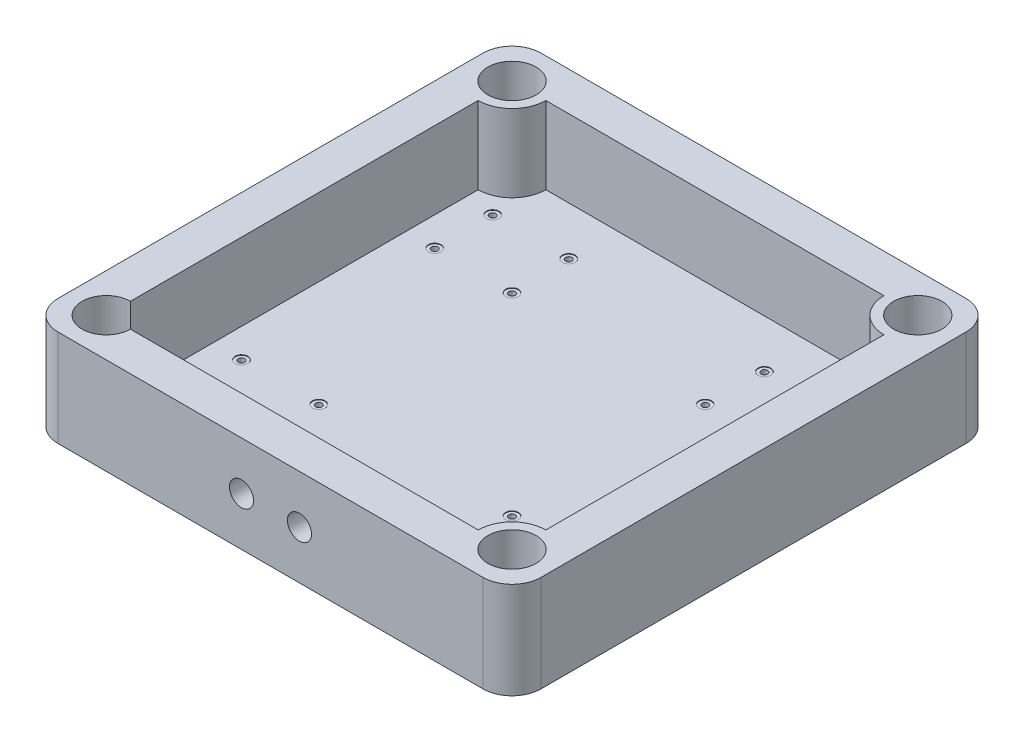
from build123d import *

# Parameters (mm, degrees)
BOSS_EXTRUDE1_DEPTH                          = 100
CUT_EXTRUDE1_DEPTH                           = 80
SKETCH3_R                                    = 25
CUT_EXTRUDE2_DEPTH                           = 80
SKETCH10_R                                   = 12.5
CUT_EXTRUDE4_DEPTH                           = 40
CBORE_FOR_M6_HEXAGON_HEAD_BOLTS_FULL_2_COUNT = 2
CBORE_FOR_M6_HEXAGON_HEAD_BOLTS_FULL_2_PITCH = 80
CBORE_FOR_M6_HEXAGON_HEAD_BOLTS_FULL_3_COUNT = 2
CBORE_FOR_M6_HEXAGON_HEAD_BOLTS_FULL_3_PITCH = 60
CBORE_FOR_M6_HEXAGON_HEAD_BOLTS_FULL_4_COUNT = 2
CBORE_FOR_M6_HEXAGON_HEAD_BOLTS_FULL_4_PITCH = 98.990867508
CUT_EXTRUDE5_DEPTH                           = 80


with BuildPart() as part:
    # Sketch1 → Boss-Extrude1 (new body)
    with BuildSketch(Plane(origin=(0, 0, 0), x_dir=(1, 0, 0), z_dir=(0, 1, 0))):
        with BuildLine():
            Line((-220, -250), (220, -250))
            ThreePointArc((220, -250), (241.213203436, -241.213203436), (250, -220))
            Line((250, -220), (250, 220))
            ThreePointArc((250, 220), (241.213203436, 241.213203436), (220, 250))
            Line((220, 250), (-220, 250))
            ThreePointArc((-220, 250), (-241.213203436, 241.213203436), (-250, 220))
            Line((-250, 220), (-250, -220))
            ThreePointArc((-250, -220), (-241.213203436, -241.213203436), (-220, -250))
        make_face()
    extrude(amount=BOSS_EXTRUDE1_DEPTH)

    # Sketch2 → Cut-Extrude1 (cut)
    with BuildSketch(Plane(origin=(0, 100, 0), x_dir=(1, 0, 0), z_dir=(0, 1, 0))):
        with BuildLine():
            Line((-175, -210), (175, -210))
            ThreePointArc((175, -210), (185.251262658, -185.251262658), (210, -175))
            Line((210, -175), (210, 175))
            ThreePointArc((210, 175), (185.251262658, 185.251262658), (175, 210))
            Line((175, 210), (-175, 210))
            ThreePointArc((-175, 210), (-185.251262658, 185.251262658), (-210, 175))
            Line((-210, 175), (-210, -175))
            ThreePointArc((-210, -175), (-185.251262658, -185.251262658), (-175, -210))
        make_face()
    extrude(amount=-CUT_EXTRUDE1_DEPTH, mode=Mode.SUBTRACT)

    # Sketch3 → Cut-Extrude2 (cut)
    with BuildSketch(Plane(origin=(0, 100, 0), x_dir=(1, 0, 0), z_dir=(0, 1, 0))):
        with Locations(Location((-210, 210, 0), (0, 0, 270))):
            Circle(SKETCH3_R)
        with Locations(Location((210, 210, 0), (0, 0, 90))):
            Circle(SKETCH3_R)
        with Locations(Location((210, -210, 0), (0, 0, 270))):
            Circle(SKETCH3_R)
        with Locations(Location((-210, -210, 0), (0, 0, 90))):
            Circle(SKETCH3_R)
    extrude(amount=-CUT_EXTRUDE2_DEPTH, mode=Mode.SUBTRACT)

    # Sketch10 → Cut-Extrude4 (cut)
    with BuildSketch(Plane.XY.offset(250)):
        with Locations((-30, 50)):
            Circle(SKETCH10_R)
        with Locations((30, 50)):
            Circle(SKETCH10_R)
    extrude(amount=-CUT_EXTRUDE4_DEPTH, mode=Mode.SUBTRACT)

    # Sketch12 → CBORE for M6 Hexagon head bolts-Full thread-grade C1 (revolve, cut)
    with BuildSketch(Plane(origin=(-180, 20, 100), x_dir=(0, 0, 1), z_dir=(1, 0, 0))):
        Polygon((0, 0), (0, 20), (3.3, 20), (3.3, 0.5), (6.5, 0.5), (6.5, 0.025), (6.525, 0), align=None)
    cbore_for_m6_hexagon_head_bolts_full_thr = revolve(axis=Axis((-180, 26.35, 100), (0, -1, 0)), mode=Mode.SUBTRACT)

    # CBORE for M6 Hexagon head bolts-Full 2: CBORE for M6 Hexagon head bolts-Full thread-grade C1 ×2
    with Locations(*[Vector(0.9999999861018275, 0, 0.0001667223586748534) * (i * CBORE_FOR_M6_HEXAGON_HEAD_BOLTS_FULL_2_PITCH) for i in range(1, CBORE_FOR_M6_HEXAGON_HEAD_BOLTS_FULL_2_COUNT)]):
        add(cbore_for_m6_hexagon_head_bolts_full_thr, mode=Mode.SUBTRACT)

    # CBORE for M6 Hexagon head bolts-Full 3: CBORE for M6 Hexagon head bolts-Full thread-grade C1 ×2
    with Locations(*[(0, 0, i * CBORE_FOR_M6_HEXAGON_HEAD_BOLTS_FULL_3_PITCH) for i in range(1, CBORE_FOR_M6_HEXAGON_HEAD_BOLTS_FULL_3_COUNT)]):
        add(cbore_for_m6_hexagon_head_bolts_full_thr, mode=Mode.SUBTRACT)

    # CBORE for M6 Hexagon head bolts-Full 4: CBORE for M6 Hexagon head bolts-Full thread-grade C1 ×2
    with Locations(*[Vector(0.795375864434165, 0, 0.6061165187285402) * (i * CBORE_FOR_M6_HEXAGON_HEAD_BOLTS_FULL_4_PITCH) for i in range(1, CBORE_FOR_M6_HEXAGON_HEAD_BOLTS_FULL_4_COUNT)]):
        add(cbore_for_m6_hexagon_head_bolts_full_thr, mode=Mode.SUBTRACT)

    # Mirror1: CBORE for M6 Hexagon head bolts-Full thread-grade C1 across plane
    add(cbore_for_m6_hexagon_head_bolts_full_thr.mirror(Plane.XY), mode=Mode.SUBTRACT)

    # Mirror1 copy 1 sketch → Mirror1 copy 1 (revolve, cut)
    with BuildSketch(Plane(origin=(-100.000001112, 20, -100.013337789), x_dir=(0, 0, -1), z_dir=(1, 0, 0))):
        Polygon((0, 0), (0, -20), (3.3, -20), (3.3, -0.5), (6.5, -0.5), (6.5, -0.025), (6.525, 0), align=None)
    revolve(axis=Axis((-100.000001112, 26.35, -100.013337789), (0, 1, 0)), mode=Mode.SUBTRACT)

    # Mirror1 copy 2 sketch → Mirror1 copy 2 (revolve, cut)
    with BuildSketch(Plane(origin=(-180, 20, -160), x_dir=(0, 0, -1), z_dir=(1, 0, 0))):
        Polygon((0, 0), (0, -20), (3.3, -20), (3.3, -0.5), (6.5, -0.5), (6.5, -0.025), (6.525, 0), align=None)
    revolve(axis=Axis((-180, 26.35, -160), (0, 1, 0)), mode=Mode.SUBTRACT)

    # Mirror1 copy 3 sketch → Mirror1 copy 3 (revolve, cut)
    with BuildSketch(Plane(origin=(-101.265053185, 20, -160), x_dir=(0, 0, -1), z_dir=(1, 0, 0))):
        Polygon((0, 0), (0, -20), (3.3, -20), (3.3, -0.5), (6.5, -0.5), (6.5, -0.025), (6.525, 0), align=None)
    revolve(axis=Axis((-101.265053185, 26.35, -160), (0, 1, 0)), mode=Mode.SUBTRACT)

    # Mirror1 at the second plane: CBORE for M6 Hexagon head bolts-Full thread-grade C1 across plane
    add(cbore_for_m6_hexagon_head_bolts_full_thr.mirror(Plane(origin=(0, 0, 0), x_dir=(0, 0, 1), z_dir=(1, 0, 0))), mode=Mode.SUBTRACT)

    # Mirror1 at the second plane copy 1 sketc → Mirror1 at the second plane copy 1 (revolve, cut)
    with BuildSketch(Plane(origin=(100.000001112, 20, 100.013337789), x_dir=(0, 0, 1), z_dir=(-1, 0, 0))):
        Polygon((0, 0), (0, -20), (3.3, -20), (3.3, -0.5), (6.5, -0.5), (6.5, -0.025), (6.525, 0), align=None)
    revolve(axis=Axis((100.000001112, 26.35, 100.013337789), (0, 1, 0)), mode=Mode.SUBTRACT)

    # Mirror1 at the second plane copy 2 sketc → Mirror1 at the second plane copy 2 (revolve, cut)
    with BuildSketch(Plane(origin=(180, 20, 160), x_dir=(0, 0, 1), z_dir=(-1, 0, 0))):
        Polygon((0, 0), (0, -20), (3.3, -20), (3.3, -0.5), (6.5, -0.5), (6.5, -0.025), (6.525, 0), align=None)
    revolve(axis=Axis((180, 26.35, 160), (0, 1, 0)), mode=Mode.SUBTRACT)

    # Mirror1 at the second plane copy 3 sketc → Mirror1 at the second plane copy 3 (revolve, cut)
    with BuildSketch(Plane(origin=(101.265053185, 20, 160), x_dir=(0, 0, 1), z_dir=(-1, 0, 0))):
        Polygon((0, 0), (0, -20), (3.3, -20), (3.3, -0.5), (6.5, -0.5), (6.5, -0.025), (6.525, 0), align=None)
    revolve(axis=Axis((101.265053185, 26.35, 160), (0, 1, 0)), mode=Mode.SUBTRACT)

    # Mirror1 at the second plane copy 4 sketc → Mirror1 at the second plane copy 4 (revolve, cut)
    with BuildSketch(Plane(origin=(180, 20, -100), x_dir=(0, 0, -1), z_dir=(-1, 0, 0))):
        Polygon((0, 0), (0, 20), (3.3, 20), (3.3, 0.5), (6.5, 0.5), (6.5, 0.025), (6.525, 0), align=None)
    revolve(axis=Axis((180, 26.35, -100), (0, -1, 0)), mode=Mode.SUBTRACT)

    # Mirror1 at the second plane copy 5 sketc → Mirror1 at the second plane copy 5 (revolve, cut)
    with BuildSketch(Plane(origin=(100.000001112, 20, -100.013337789), x_dir=(0, 0, -1), z_dir=(-1, 0, 0))):
        Polygon((0, 0), (0, 20), (3.3, 20), (3.3, 0.5), (6.5, 0.5), (6.5, 0.025), (6.525, 0), align=None)
    revolve(axis=Axis((100.000001112, 26.35, -100.013337789), (0, -1, 0)), mode=Mode.SUBTRACT)

    # Mirror1 at the second plane copy 6 sketc → Mirror1 at the second plane copy 6 (revolve, cut)
    with BuildSketch(Plane(origin=(180, 20, -160), x_dir=(0, 0, -1), z_dir=(-1, 0, 0))):
        Polygon((0, 0), (0, 20), (3.3, 20), (3.3, 0.5), (6.5, 0.5), (6.5, 0.025), (6.525, 0), align=None)
    revolve(axis=Axis((180, 26.35, -160), (0, -1, 0)), mode=Mode.SUBTRACT)

    # Mirror1 at the second plane copy 7 sketc → Mirror1 at the second plane copy 7 (revolve, cut)
    with BuildSketch(Plane(origin=(101.265053185, 20, -160), x_dir=(0, 0, -1), z_dir=(-1, 0, 0))):
        Polygon((0, 0), (0, 20), (3.3, 20), (3.3, 0.5), (6.5, 0.5), (6.5, 0.025), (6.525, 0), align=None)
    revolve(axis=Axis((101.265053185, 26.35, -160), (0, -1, 0)), mode=Mode.SUBTRACT)

    # Sketch14 → Cut-Extrude5 (cut)
    with BuildSketch(Plane(origin=(0, 100, 0), x_dir=(1, 0, 0), z_dir=(0, 1, 0))):
        with BuildLine():
            Line((-210, -175), (-210, -210))
            Line((-210, -210), (-175, -210))
            ThreePointArc((-175, -210), (-185.251262658, -185.251262658), (-210, -175))
        make_face()
    extrude(amount=-CUT_EXTRUDE5_DEPTH, mode=Mode.SUBTRACT)


solid = part.part
